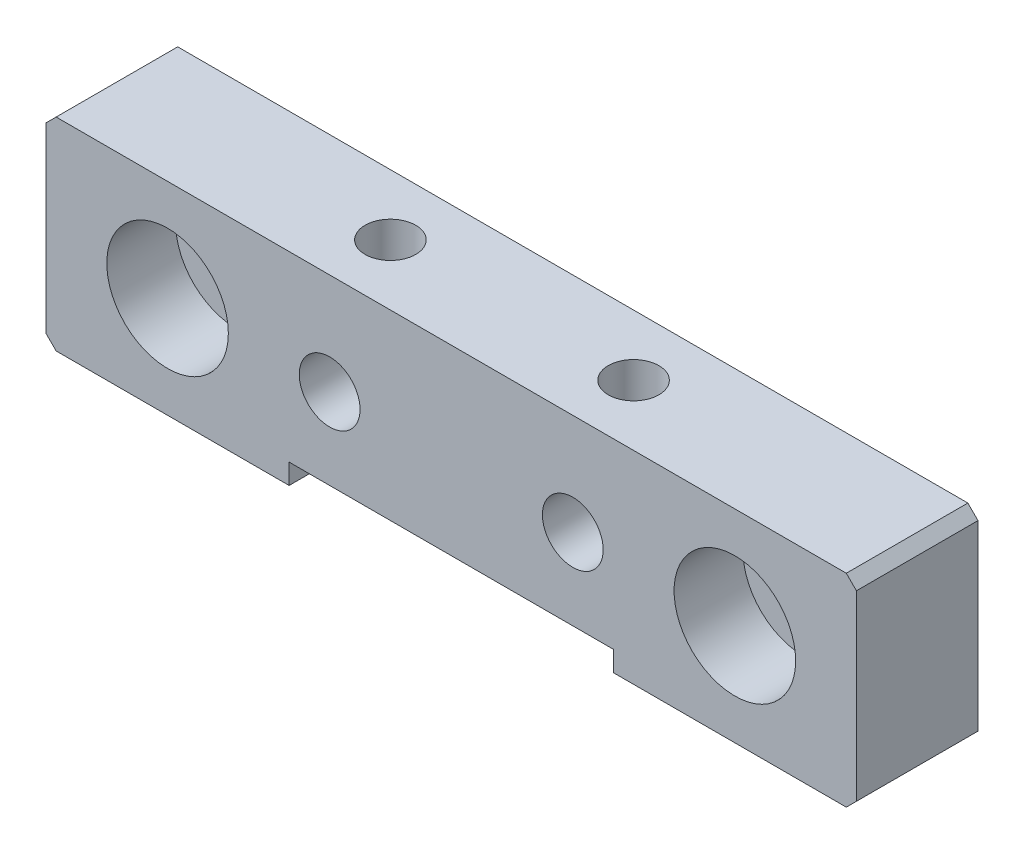
from build123d import *

# Parameters (mm, degrees)
SKETCH1_W                                            = 40
SKETCH1_H                                            = 10
BOSS_EXTRUDE1_DEPTH                                  = 6
CHAMFER1_SIZE                                        = 0.5
HOLE_SIZE_PER_SOCKET_HEAD_CAP_SCREW_TYPE_D           = 3.4
HOLE_SIZE_PER_SOCKET_HEAD_CAP_SCREW_TYPE_CBORE_D     = 6
HOLE_SIZE_PER_SOCKET_HEAD_CAP_SCREW_TYPE_CBORE_DEPTH = 3.4
SKETCH4_W                                            = 16
SKETCH4_H                                            = 6
CUT_EXTRUDE1_DEPTH                                   = 1
SKETCH5_R                                            = 1.5
CUT_EXTRUDE2_DEPTH                                   = 22.470910554
M3_TAPPED_HOLE1_D                                    = 2.5
M3_TAPPED_HOLE1_DEPTH                                = 5
M3_TAPPED_HOLE1_TIP                                  = 0.751075774


with BuildPart() as part:
    # Sketch1 → Boss-Extrude1 (new body)
    with BuildSketch(Plane.XY):
        Rectangle(SKETCH1_W, SKETCH1_H)
    extrude(amount=BOSS_EXTRUDE1_DEPTH)

    # Chamfer1
    chamfer1_edges = [part.edges().sort_by_distance(p)[0] for p in [
        (-20, 5, 3),
        (20, 5, 3),
        (20, -5, 3),
        (-20, -5, 3),
    ]]
    chamfer(chamfer1_edges, length=CHAMFER1_SIZE)

    # Hole Size per Socket Head Cap Screw Type1 (through all)
    with Locations(Plane.XY.offset(6)):
        with Locations((-14, 0), (14, 0)):
            CounterBoreHole(HOLE_SIZE_PER_SOCKET_HEAD_CAP_SCREW_TYPE_D / 2, HOLE_SIZE_PER_SOCKET_HEAD_CAP_SCREW_TYPE_CBORE_D / 2, HOLE_SIZE_PER_SOCKET_HEAD_CAP_SCREW_TYPE_CBORE_DEPTH)

    # Sketch4 → Cut-Extrude1 (cut)
    with BuildSketch(Plane(origin=(0, -5, 0), x_dir=(1, 0, 0), z_dir=(0, 1, 0))):
        with Locations((0, -3)):
            Rectangle(SKETCH4_W, SKETCH4_H)
    extrude(amount=CUT_EXTRUDE1_DEPTH, mode=Mode.SUBTRACT)

    # Sketch5 → Cut-Extrude2 (cut, through all)
    with BuildSketch(Plane.XY):
        with Locations((-6, 0)):
            Circle(SKETCH5_R)
        with Locations((6, 0)):
            Circle(SKETCH5_R)
    extrude(amount=CUT_EXTRUDE2_DEPTH, mode=Mode.SUBTRACT)

    # M3 Tapped Hole1
    with Locations(Plane(origin=(0, 5, 0), x_dir=(-1, 0, 0), z_dir=(0, 1, 0))):
        with Locations((6, 3), (-6, 3)):
            Hole(M3_TAPPED_HOLE1_D / 2, depth=M3_TAPPED_HOLE1_DEPTH)
            with Locations((0, 0, -(M3_TAPPED_HOLE1_DEPTH + M3_TAPPED_HOLE1_TIP / 2))):  # 118° drill point
                Cone(0, M3_TAPPED_HOLE1_D / 2, M3_TAPPED_HOLE1_TIP, mode=Mode.SUBTRACT)


solid = part.part
